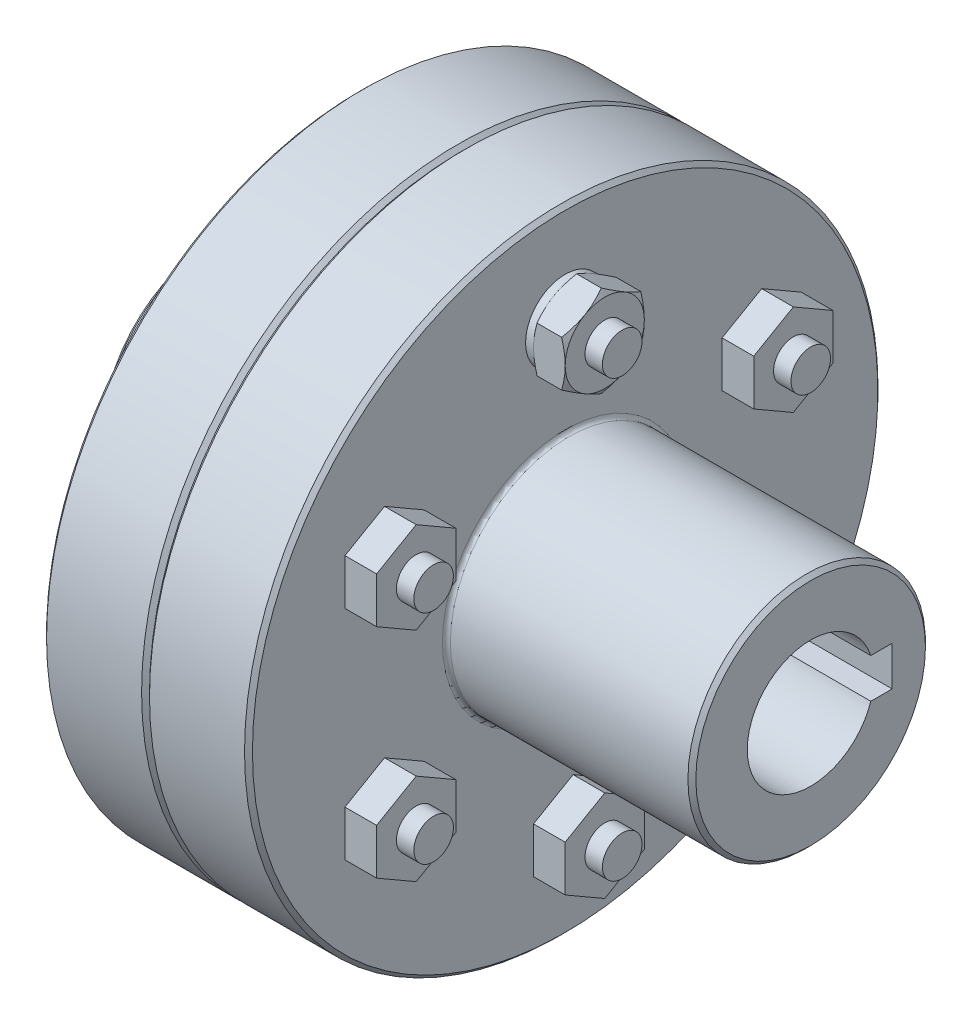
from build123d import *

# Parameters (mm, degrees)
CHAMFER_1_SIZE                       = 0.5
CHAMFER_2_SIZE                       = 0.5
FILLET_1_R                           = 1
CUT_EXTRUDE_5_DEPTH                  = 65.505813691
CUT_EXTRUDE_5_DEPTH_BACK             = 65.505813691
SKETCH_15_R                          = 6
CUT_EXTRUDE_7_DEPTH                  = 65.505813691
CUT_EXTRUDE_7_DEPTH_BACK             = 65.505813691
SKETCH_16_R                          = 8
CUT_EXTRUDE_6_DEPTH                  = 72.665891469
CUT_EXTRUDE_10_DEPTH                 = 72.665891469
CHAMFER_3_SIZE                       = 0.5
CHAMFER_4_SIZE                       = 0.5
FILLET_2_R                           = 0.5
SKETCH_6_R                           = 2.5
CUT_EXTRUDE_1_DEPTH                  = 26
CHAMFER_5_SIZE                       = 0.2
CHAMFER_6_SIZE                       = 0.2
PATTERN_CIRCULAR_1_COUNT             = 6
CHAMFER_5_OF_PATTERN_CIRCULAR_1_SIZE = 0.2
CHAMFER_6_OF_PATTERN_CIRCULAR_1_SIZE = 0.2
SKETCH_7_W                           = 33.2
SKETCH_7_H                           = 2.5
EXTRUDE_1_DEPTH                      = 4
SKETCH_9_R                           = 7.5
SKETCH_9_R_2                         = 5
CUT_EXTRUDE_2_DEPTH                  = 1
CUT_EXTRUDE_2_DRAFT                  = -60
SKETCH_10_R                          = 5
EXTRUDE_2_DEPTH                      = 1
EXTRUDE_3_DEPTH                      = 4
SKETCH_12_R                          = 7.5
SKETCH_12_R_2                        = 5
CUT_EXTRUDE_3_DEPTH                  = 1
CUT_EXTRUDE_3_DRAFT                  = -60
SKETCH_13_R                          = 7.5
SKETCH_13_R_2                        = 5
CUT_EXTRUDE_4_DEPTH                  = 1
CUT_EXTRUDE_4_DRAFT                  = -60
PATTERN_CIRCULAR_2_COUNT             = 6
CUT_EXTRUDE_15_REACH                 = 95.941
SKETCH_29_R                          = 7


with BuildPart() as part:
    # 草图2 → 旋转1 (revolve)
    with BuildSketch(Plane.XY, mode=Mode.PRIVATE) as revolve_1_sk:
        Polygon((-31, 15), (-31, 0), (1, 0), (1, 15), (0, 15), (0, 40), (-13, 40), (-13, 15), align=None)
    revolve(revolve_1_sk.sketch.rotate(Axis((-31, 0, 0), (1, 0, 0)), 90), axis=Axis((-31, 0, 0), (1, 0, 0)))

    # 倒角1
    chamfer_1_edges = [part.edges().sort_by_distance(p)[0] for p in [
        (-31, 0, -15),
    ]]
    chamfer(chamfer_1_edges, length=CHAMFER_1_SIZE)

    # 倒角2
    chamfer_2_edges = [part.edges().sort_by_distance(p)[0] for p in [
        (-13, 0, -40),
        (0, 0, -40),
    ]]
    chamfer(chamfer_2_edges, length=CHAMFER_2_SIZE)

    # 圆角1
    fillet_1_edges = [part.edges().sort_by_distance(p)[0] for p in [
        (-13, 0, -15),
    ]]
    fillet(fillet_1_edges, radius=FILLET_1_R)

    # 草图15 → 切除-拉伸5 (cut, two sides: drawn at the far end of the back side and taken through both)
    with BuildSketch(Plane(origin=(0, 0, 0), x_dir=(0, 0, -1), z_dir=(1, 0, 0)).offset(-CUT_EXTRUDE_5_DEPTH_BACK)):
        Circle(SKETCH_15_R)
    extrude(amount=CUT_EXTRUDE_5_DEPTH + CUT_EXTRUDE_5_DEPTH_BACK, mode=Mode.SUBTRACT)

    # 草图20 → 切除-拉伸7 (cut, two sides: drawn at the far end of the back side and taken through both)
    with BuildSketch(Plane(origin=(0, 0, 0), x_dir=(0, 0, -1), z_dir=(1, 0, 0)).offset(-CUT_EXTRUDE_7_DEPTH_BACK)):
        with BuildLine():
            Line((7.8, -2), (7.8, 2))
            Line((7.8, 2), (5.656854249, 2))
            ThreePointArc((5.656854249, 2), (5.913591358, 1.014611872), (6, 0))
            ThreePointArc((6, 0), (5.913591358, -1.014611872), (5.656854249, -2))
            Line((5.656854249, -2), (7.8, -2))
        make_face()
    extrude(amount=CUT_EXTRUDE_7_DEPTH + CUT_EXTRUDE_7_DEPTH_BACK, mode=Mode.SUBTRACT)


with BuildPart() as body_2:
    # 草图3 → 旋转2 (revolve)
    with BuildSketch(Plane.XY, mode=Mode.PRIVATE) as revolve_2_sk:
        Polygon((13, 40), (0, 40), (0, 15), (2, 15), (2, 0), (44, 0), (44, 8), (44, 15), (13, 15), align=None)
    revolve(revolve_2_sk.sketch.rotate(Axis((-31, 0, 0), (1, 0, 0)), 270), axis=Axis((-31, 0, 0), (1, 0, 0)))

    # 草图16 → 切除-拉伸6 (cut, through all)
    with BuildSketch(Plane(origin=(0, 0, 0), x_dir=(0, 0, -1), z_dir=(1, 0, 0))):
        Circle(SKETCH_16_R)
    extrude(amount=CUT_EXTRUDE_6_DEPTH, mode=Mode.SUBTRACT)

    # 草图24 → 切除-拉伸10 (cut, through all)
    with BuildSketch(Plane(origin=(0, 0, 0), x_dir=(0, 0, -1), z_dir=(1, 0, 0))):
        with BuildLine():
            Line((10.3, -2.5), (10.3, 2.5))
            Line((10.3, 2.5), (7.599342077, 2.5))
            ThreePointArc((7.599342077, 2.5), (7.899200485, 1.265950905), (8, 0))
            ThreePointArc((8, 0), (7.899200485, -1.265950905), (7.599342077, -2.5))
            Line((7.599342077, -2.5), (10.3, -2.5))
        make_face()
    extrude(amount=CUT_EXTRUDE_10_DEPTH, mode=Mode.SUBTRACT)

    # 倒角3
    chamfer_3_edges = [body_2.edges().sort_by_distance(p)[0] for p in [
        (13, 0, 40),
        (0, 0, 40),
    ]]
    chamfer(chamfer_3_edges, length=CHAMFER_3_SIZE)

    # 倒角4
    chamfer_4_edges = [body_2.edges().sort_by_distance(p)[0] for p in [
        (44, 0, 15),
    ]]
    chamfer(chamfer_4_edges, length=CHAMFER_4_SIZE)

    # 圆角2
    fillet_2_edges = [body_2.edges().sort_by_distance(p)[0] for p in [
        (13, 0, 15),
    ]]
    fillet(fillet_2_edges, radius=FILLET_2_R)


with BuildPart() as cut_extrude_1_tool:
    # 草图6 → 切除-拉伸1 (new body)
    with BuildSketch(Plane.ZY.offset(13)):
        with Locations((0, 27.5)):
            Circle(SKETCH_6_R)
    cut_extrude_1 = extrude(amount=-CUT_EXTRUDE_1_DEPTH)


with BuildPart() as part_1:
    add(part.part)

    # 切除-拉伸1: cut by cut_extrude_1_tool
    add(cut_extrude_1_tool.part, mode=Mode.SUBTRACT)

    # 倒角5
    chamfer_5_edges = [part_1.edges().sort_by_distance(p)[0] for p in [
        (-13, 27.5, -2.5),
    ]]
    chamfer(chamfer_5_edges, length=CHAMFER_5_SIZE)


with BuildPart() as body_2_1:
    add(body_2.part)

    # 切除-拉伸1: cut by cut_extrude_1_tool
    add(cut_extrude_1_tool.part, mode=Mode.SUBTRACT)

    # 倒角6
    chamfer_6_edges = [body_2_1.edges().sort_by_distance(p)[0] for p in [
        (13, 27.5, -2.5),
    ]]
    chamfer(chamfer_6_edges, length=CHAMFER_6_SIZE)


with BuildPart() as pattern_circular_1_tool:
    # 阵列(圆周)1: 切除-拉伸1 ×6 about axis
    pattern_circular_1_axis = Axis((0, 0, 0), (1, 0, 0))
    for i in range(1, PATTERN_CIRCULAR_1_COUNT):
        add(cut_extrude_1.rotate(pattern_circular_1_axis, i * 360 / PATTERN_CIRCULAR_1_COUNT))


with BuildPart() as part_2:
    add(part_1.part)

    # 阵列(圆周)1: cut by pattern_circular_1_tool
    add(pattern_circular_1_tool.part, mode=Mode.SUBTRACT)

    # 倒角5 of 阵列(圆周)1
    chamfer_5_of_pattern_circular_1_edges = [part_2.edges().sort_by_distance(p)[0] for p in [
        (-13, 15.915063509, 22.565698604),
        (-13, -11.584936491, 25.065698604),
        (-13, -27.5, 2.5),
        (-13, -15.915063509, -22.565698604),
        (-13, 11.584936491, -25.065698604),
    ]]
    chamfer(chamfer_5_of_pattern_circular_1_edges, length=CHAMFER_5_OF_PATTERN_CIRCULAR_1_SIZE)



with BuildPart() as body_2_2:
    add(body_2_1.part)

    # 阵列(圆周)1: cut by pattern_circular_1_tool
    add(pattern_circular_1_tool.part, mode=Mode.SUBTRACT)

    # 倒角6 of 阵列(圆周)1
    chamfer_6_of_pattern_circular_1_edges = [body_2_2.edges().sort_by_distance(p)[0] for p in [
        (13, 15.915063509, 22.565698604),
        (13, -11.584936491, 25.065698604),
        (13, -27.5, 2.5),
        (13, -15.915063509, -22.565698604),
        (13, 11.584936491, -25.065698604),
    ]]
    chamfer(chamfer_6_of_pattern_circular_1_edges, length=CHAMFER_6_OF_PATTERN_CIRCULAR_1_SIZE)


with BuildPart() as part_3:
    add(part_2.part)

    add(body_2_2.part)  # 旋转3 merges body 2
    # 草图7 → 旋转3 (revolve)
    with BuildSketch(Plane.XY, mode=Mode.PRIVATE) as revolve_3_sk:
        with Locations((3.6, 28.75)):
            Rectangle(SKETCH_7_W, SKETCH_7_H)
    revolve_3 = revolve(revolve_3_sk.sketch.rotate(Axis((20.2, 27.5, 0), (-1, 0, 0)), 90), axis=Axis((20.2, 27.5, 0), (-1, 0, 0)))

    # 草图8 → 凸台-拉伸1 (add)
    with BuildSketch(Plane.ZY.offset(13)):
        Polygon((0, 33.273502692), (-5, 30.386751346), (-5, 24.613248654), (0, 21.726497308), (5, 24.613248654), (5, 30.386751346), align=None)
    extrude_1 = extrude(amount=EXTRUDE_1_DEPTH)


with BuildPart() as cut_extrude_2_tool:
    # 草图9 → 切除-拉伸2 (with draft: the straight prism first)
    with BuildSketch(Plane.ZY.offset(17)):
        with Locations((0, 27.5)):
            Circle(SKETCH_9_R)
        with Locations((0, 27.5)):
            Circle(SKETCH_9_R_2, mode=Mode.SUBTRACT)
    extrude(amount=-CUT_EXTRUDE_2_DEPTH)
    # 切除-拉伸2: the draft: its side faces are tilted about the plane it starts from
    cut_extrude_2_sides = [cut_extrude_2_tool.faces().sort_by_distance(p)[0] for p in [
        (-16.5, 27.5, -7.5),
        (-16.5, 27.5, -5),
    ]]
    draft(cut_extrude_2_sides, Plane.ZY.offset(17), CUT_EXTRUDE_2_DRAFT)


with BuildPart() as part_4:
    add(part_3.part)

    # 切除-拉伸2: cut by cut_extrude_2_tool
    add(cut_extrude_2_tool.part, mode=Mode.SUBTRACT)

    # 草图10 → 凸台-拉伸2 (add)
    with BuildSketch(Plane(origin=(13, 0, 0), x_dir=(0, 0, -1), z_dir=(1, 0, 0))):
        with Locations(Location((0, 27.5, 0), (0, 0, 180))):
            Circle(SKETCH_10_R)
    extrude(amount=EXTRUDE_2_DEPTH)

    # 草图11 → 凸台-拉伸3 (add)
    with BuildSketch(Plane(origin=(14, 0, 0), x_dir=(0, 0, -1), z_dir=(1, 0, 0))):
        Polygon((5, 30.386751346), (0, 33.273502692), (-5, 30.386751346), (-5, 24.613248654), (0, 21.726497308), (5, 24.613248654), align=None)
    extrude_3 = extrude(amount=EXTRUDE_3_DEPTH)


with BuildPart() as cut_extrude_3_tool:
    # 草图12 → 切除-拉伸3 (with draft: the straight prism first)
    with BuildSketch(Plane(origin=(18, 0, 0), x_dir=(0, 0, -1), z_dir=(1, 0, 0))):
        with Locations((0, 27.5)):
            Circle(SKETCH_12_R)
        with Locations(Location((0, 27.5, 0), (0, 0, 180))):
            Circle(SKETCH_12_R_2, mode=Mode.SUBTRACT)
    extrude(amount=-CUT_EXTRUDE_3_DEPTH)
    # 切除-拉伸3: the draft: its side faces are tilted about the plane it starts from
    cut_extrude_3_sides = [cut_extrude_3_tool.faces().sort_by_distance(p)[0] for p in [
        (17.5, 27.5, 7.5),
        (17.5, 27.5, -5),
    ]]
    draft(cut_extrude_3_sides, Plane(origin=(18, 0, 0), x_dir=(0, 0, -1), z_dir=(1, 0, 0)), CUT_EXTRUDE_3_DRAFT)


with BuildPart() as part_5:
    add(part_4.part)

    # 切除-拉伸3: cut by cut_extrude_3_tool
    add(cut_extrude_3_tool.part, mode=Mode.SUBTRACT)


with BuildPart() as cut_extrude_4_tool:
    # 草图13 → 切除-拉伸4 (with draft: the straight prism first)
    with BuildSketch(Plane.ZY.offset(-14)):
        with Locations((0, 27.5)):
            Circle(SKETCH_13_R)
        with Locations((0, 27.5)):
            Circle(SKETCH_13_R_2, mode=Mode.SUBTRACT)
    extrude(amount=-CUT_EXTRUDE_4_DEPTH)
    # 切除-拉伸4: the draft: its side faces are tilted about the plane it starts from
    cut_extrude_4_sides = [cut_extrude_4_tool.faces().sort_by_distance(p)[0] for p in [
        (14.5, 27.5, -7.5),
        (14.5, 27.5, -5),
    ]]
    draft(cut_extrude_4_sides, Plane.ZY.offset(-14), CUT_EXTRUDE_4_DRAFT)


with BuildPart() as part_6:
    add(part_5.part)

    # 切除-拉伸4: cut by cut_extrude_4_tool
    add(cut_extrude_4_tool.part, mode=Mode.SUBTRACT)

    # 阵列(圆周)2: 旋转3, 凸台-拉伸1, 凸台-拉伸3 ×6 about axis
    pattern_circular_2_axis = Axis((0, 0, 0), (1, 0, 0))
    add([revolve_3.rotate(pattern_circular_2_axis, i * 360 / PATTERN_CIRCULAR_2_COUNT) for i in range(1, PATTERN_CIRCULAR_2_COUNT)])
    add([extrude_1.rotate(pattern_circular_2_axis, i * 360 / PATTERN_CIRCULAR_2_COUNT) for i in range(1, PATTERN_CIRCULAR_2_COUNT)])
    add([extrude_3.rotate(pattern_circular_2_axis, i * 360 / PATTERN_CIRCULAR_2_COUNT) for i in range(1, PATTERN_CIRCULAR_2_COUNT)])

    # 草图29 → 切除-拉伸15 (cut, up to next)
    with BuildSketch(Plane.ZY.offset(31), mode=Mode.PRIVATE) as cut_extrude_15_sk1:
        Circle(SKETCH_29_R)
    cut_extrude_15_tool1 = extrude(cut_extrude_15_sk1.sketch, amount=-CUT_EXTRUDE_15_REACH, mode=Mode.PRIVATE) & part_6.part
    add(cut_extrude_15_tool1.solids().sort_by_distance((-31, 0, 0))[0], mode=Mode.SUBTRACT)


solid = part_6.part
